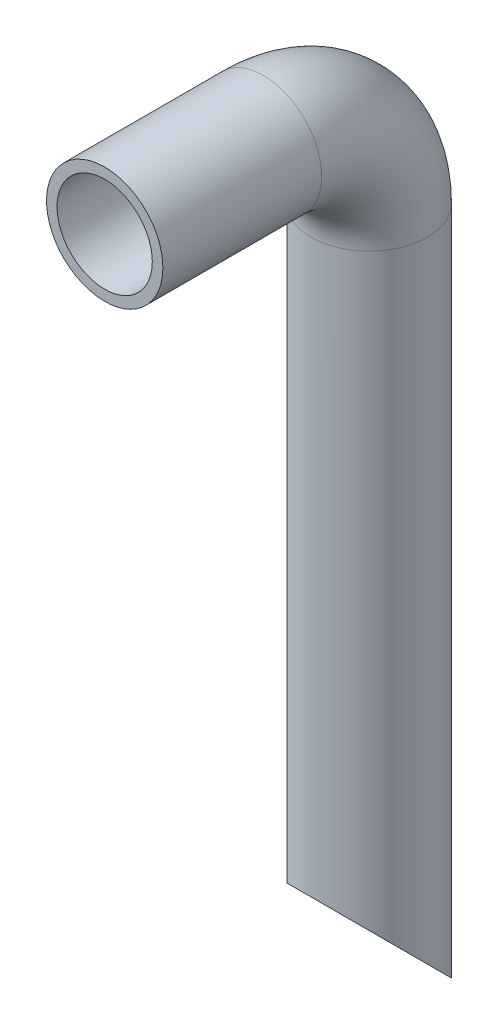
SolidWorks part; units mm, degrees
ref_plane "Front Plane" through (0, 0, 0) normal (0, 0, 1) x (1, 0, 0)
ref_plane "Top Plane" through (0, 0, 0) normal (0, 1, 0) x (1, 0, 0)
ref_plane "Right Plane" through (0, 0, 0) normal (1, 0, 0) x (0, 0, -1)
sketch "Sketch1" plane through (0, 0, 0) normal (0, 0, 1) x (1, 0, 0)
  line L0 (0, -12.1) -> (0, 12.1) construction
  circle A0 centre (0, 0) radius 11
  circle A1 centre (0, 0) radius 9
  dimension "D1" = 22
  dimension "D2" = 18
sketch "Sketch2" plane through (0, 0, 0) normal (1, 0, 0) x (0, 0, -1)
  line L0 (0, 0) -> (30, 0)
  line L1 (0, 11) -> (0, -11) construction
  line L2 (50, -20) -> (50, -150)
  arc A0 (30, 0) -> (50, -20) centre (30, -20) cw
  point P7 (50, 0)
  dimension "D3" = 20
  dimension "D1" = 50
  dimension "D2" = 150
sweep "Sweep1" add profiles "Sketch1" path "Sketch2"
sketch "Sketch3" plane through (0, 0, 0) normal (1, 0, 0) x (0, 0, -1)
  line L0 (61, -150) -> (36.2444, -125.2444)
  line L2 (61, -150) -> (36.2444, -150)
  line L3 (36.2444, -150) -> (36.2444, -125.2444)
  dimension "D1" = 45
extrude "Cut-Extrude1" cut sketch "Sketch3" against normal mid plane 50
